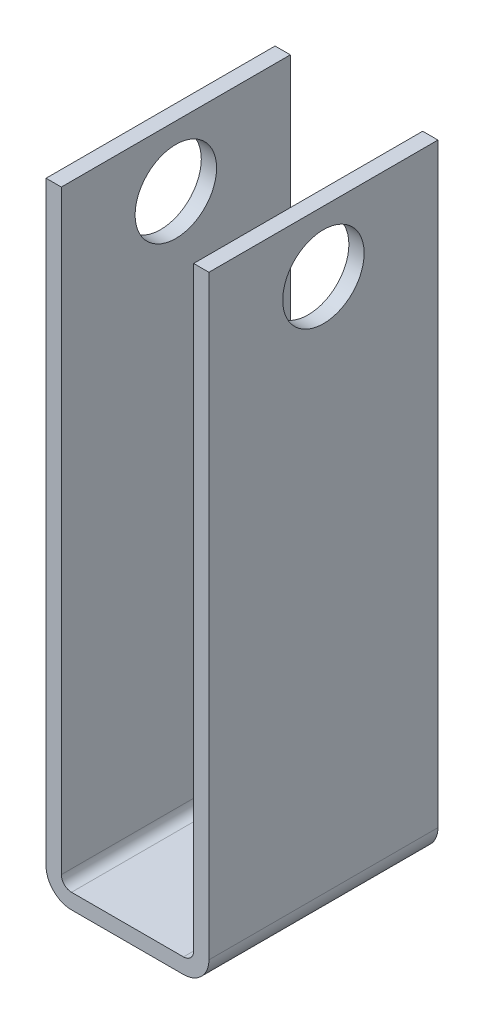
from build123d import *

# Parameters (mm, degrees)
BOSS_EXTRUDE1_DEPTH = 45
SKETCH2_R           = 8
CUT_EXTRUDE1_DEPTH  = 134.914151605


with BuildPart() as part:
    # Sketch1 → Boss-Extrude1 (new body)
    with BuildSketch(Plane.XY):
        with BuildLine():
            Line((0, 0), (0, -117))
            ThreePointArc((0, -117), (1.464466094, -120.535533906), (5, -122))
            Line((5, -122), (27, -122))
            ThreePointArc((27, -122), (30.535533906, -120.535533906), (32, -117))
            Line((32, -117), (32, 0))
            Line((32, 0), (29, 0))
            Line((29, 0), (29, -117))
            ThreePointArc((29, -117), (28.414213562, -118.414213562), (27, -119))
            Line((27, -119), (5, -119))
            ThreePointArc((5, -119), (3.585786438, -118.414213562), (3, -117))
            Line((3, -117), (3, 0))
            Line((3, 0), (0, 0))
        make_face()
    extrude(amount=BOSS_EXTRUDE1_DEPTH)

    # Sketch2 → Cut-Extrude1 (cut, through all)
    with BuildSketch(Plane(origin=(32, 0, 0), x_dir=(0, 0, -1), z_dir=(1, 0, 0))):
        with Locations((-22.5, -12)):
            Circle(SKETCH2_R)
    extrude(amount=-CUT_EXTRUDE1_DEPTH, mode=Mode.SUBTRACT)


solid = part.part
